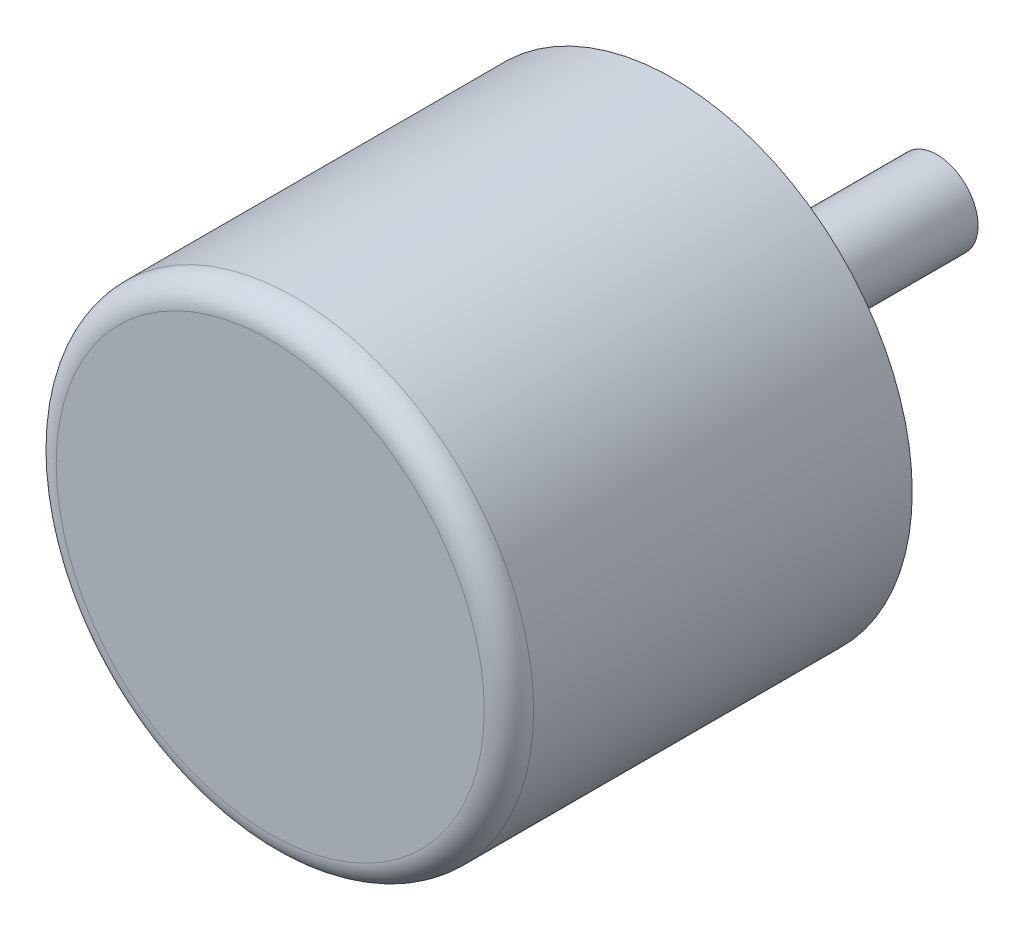
SolidWorks part; units mm, degrees
ref_plane "Front" through (0, 0, 0) normal (0, 0, 1) x (1, 0, 0)
ref_plane "Top" through (0, 0, 0) normal (0, 1, 0) x (1, 0, 0)
ref_plane "Right" through (0, 0, 0) normal (1, 0, 0) x (0, 0, -1)
sketch "草图1" plane through (0, 0, 0) normal (0, 0, 1) x (1, 0, 0)
  circle A0 centre (0, 0) radius 29
  dimension "D1" = 58
extrude "凸台-拉伸1" add sketch "草图1" along normal mid plane 49
fillet "圆角1" radius 3 1 edges at (29, 0, 24.5)
sketch "草图2" plane through (0, 0, -24.5) normal (0, 0, -1) x (-1, 0, 0)
  circle A0 centre (0, 0) radius 5
  dimension "D1" = 10
extrude "凸台-拉伸2" add sketch "草图2" along normal blind 32
hole_wizard "M3 螺纹孔1" positions "草图4" profile "草图3" tap size "M3" standard "Gb"
sketch "草图4" plane through (0, 0, -24.5) normal (0, 0, -1) x (-1, 0, 0)
  circle A0 centre (0, 0) radius 24 construction
  point P0 (24, 0)
  dimension "D1" = 48
sketch "草图3" plane through (-24, 0, -24.5) normal (1, 0, 0) x (0, 1, 0)
  line L0 (0, 0) -> (0, 8.2511)
  line L1 (0, 8.2511) -> (1.25, 7.5)
  line L2 (1.25, 7.5) -> (1.25, 0)
  line L5 (1.25, 0) -> (0, 0)
  line L10 (0, 8.2511) -> (-1.25, 7.5) construction
  line L11 (0, -6.35) -> (0, 107.95) construction
  dimension "螺纹孔钻头直径" = 2.5
  dimension "螺纹孔钻头深度" = 7.5
  dimension "导头角度" = 118
cosmetic thread "孔螺蚊线1" parameters "D1"=6, "D2"=3
pattern_circular "阵列(圆周)1" count 3 over 360 about axis through (0, 0, 0) along (0, 0, 1) of "M3 螺纹孔1"
sketch "草图5" plane through (0, 0, -24.5) normal (0, 0, -1) x (-1, 0, 0)
  circle A0 centre (0, 0) radius 18
  dimension "D1" = 36
extrude "凸台-拉伸3" add sketch "草图5" along normal blind 2.5
